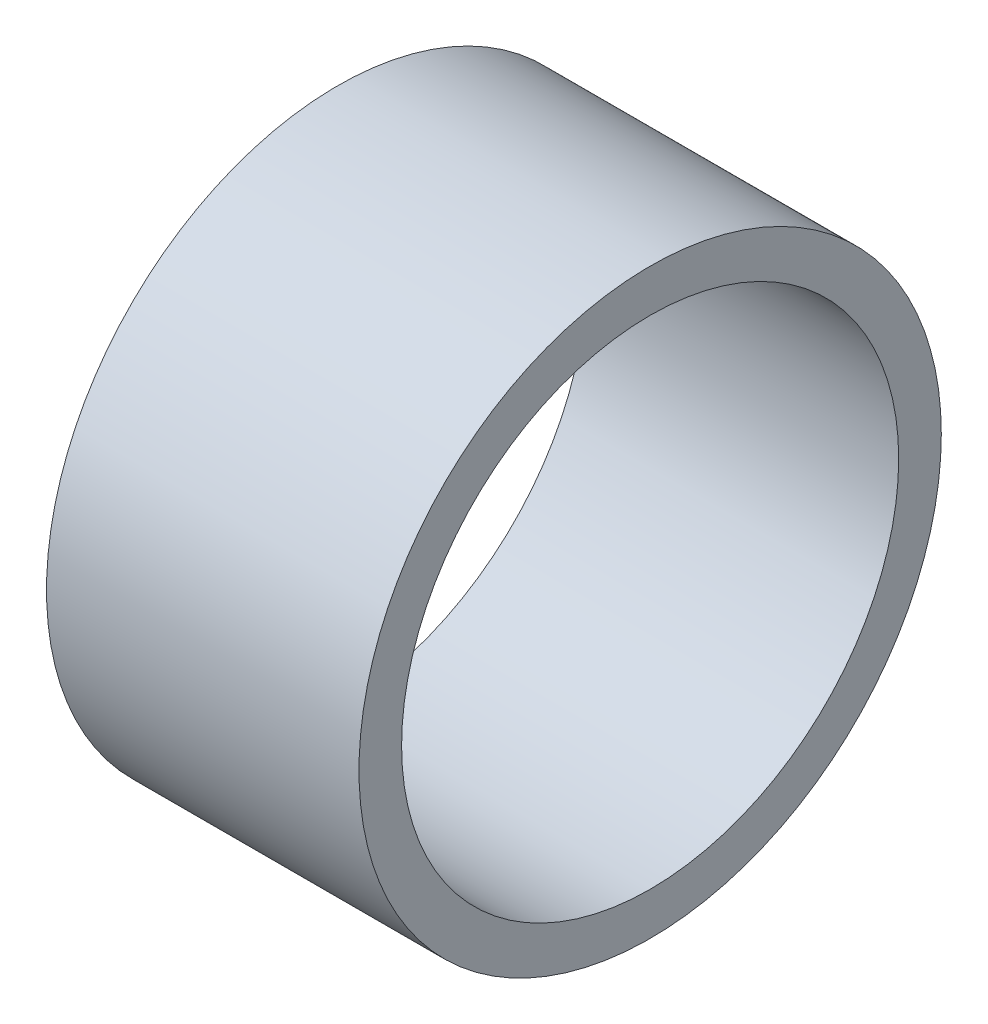
SolidWorks part; units mm, degrees
ref_plane "前视基准面" through (0, 0, 0) normal (0, 0, 1) x (1, 0, 0)
ref_plane "上视基准面" through (0, 0, 0) normal (0, 1, 0) x (1, 0, 0)
ref_plane "右视基准面" through (0, 0, 0) normal (1, 0, 0) x (0, 0, -1)
sketch "草图1" plane through (0, 0, 0) normal (1, 0, 0) x (0, 0, -1)
  circle A0 centre (0, 0) radius 20.5
  circle A1 centre (0, 0) radius 17.5
extrude "凸台-拉伸1" add sketch "草图1" along normal blind 22
